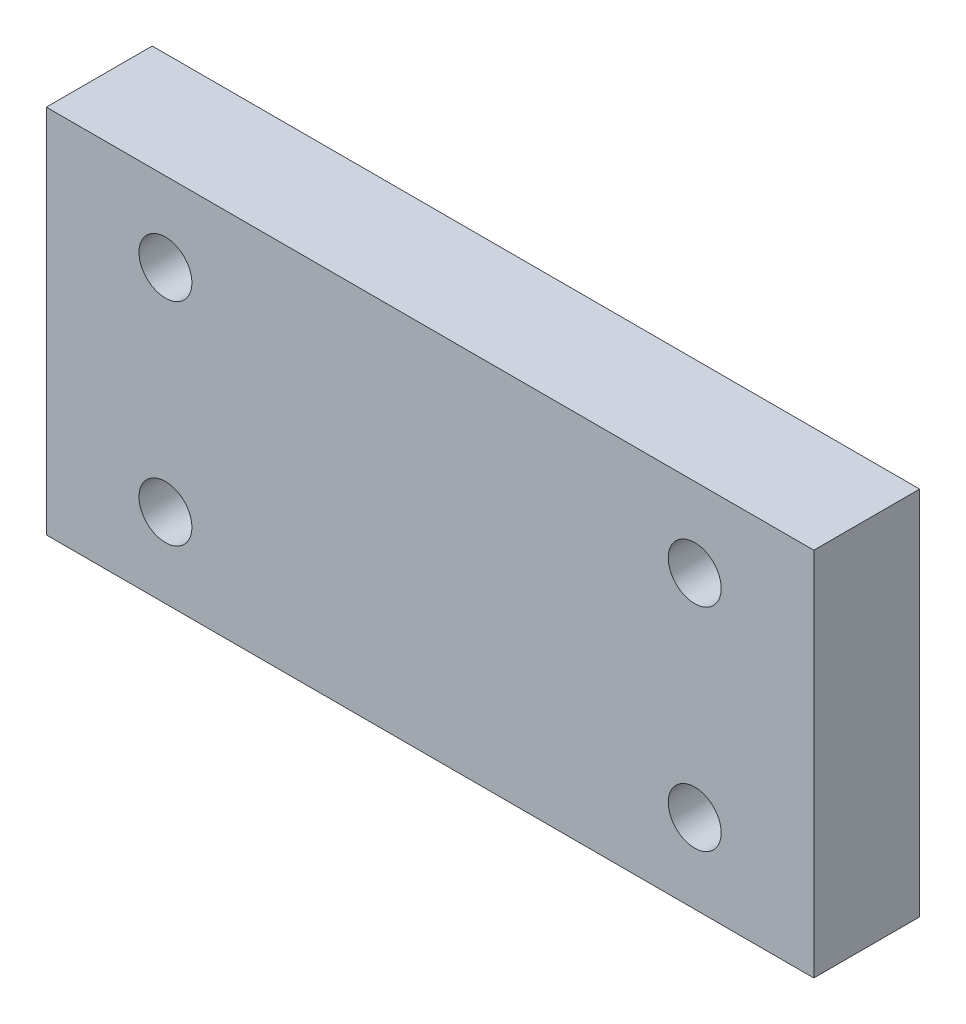
from build123d import *

# Parameters (mm, degrees)
SKETCH1_W           = 290
SKETCH1_H           = 140
SKETCH1_R           = 10
BOSS_EXTRUDE1_DEPTH = 40


with BuildPart() as part:
    # Sketch1 → Boss-Extrude1 (new body)
    with BuildSketch(Plane.XY):
        Rectangle(SKETCH1_W, SKETCH1_H)
        with Locations((-100, 40)):
            Circle(SKETCH1_R, mode=Mode.SUBTRACT)
        with Locations((-100, -40)):
            Circle(SKETCH1_R, mode=Mode.SUBTRACT)
        with Locations(Location((100, -40, 0), (0, 0, 180))):
            Circle(SKETCH1_R, mode=Mode.SUBTRACT)
        with Locations(Location((100, 40, 0), (0, 0, 180))):
            Circle(SKETCH1_R, mode=Mode.SUBTRACT)
    extrude(amount=BOSS_EXTRUDE1_DEPTH)


solid = part.part
